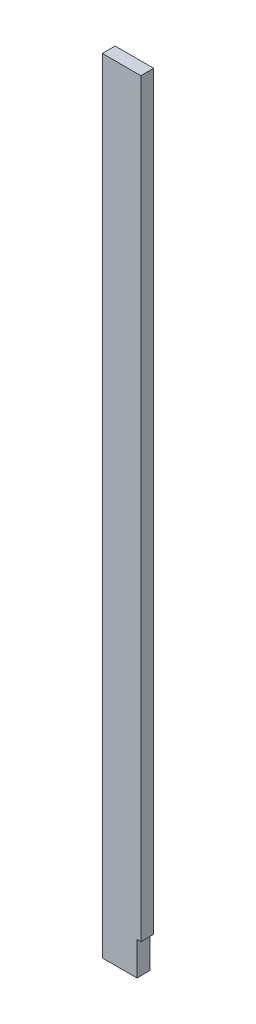
from build123d import *

# Parameters (mm, degrees)
SKETCH1_W           = 30
SKETCH1_H           = 610
BOSS_EXTRUDE1_DEPTH = 10
SKETCH2_W           = 3
SKETCH2_H           = 26
CUT_EXTRUDE1_DEPTH  = 10


with BuildPart() as part:
    # Sketch1 → Boss-Extrude1 (new body)
    with BuildSketch(Plane.XY):
        with Locations((15, -305)):
            Rectangle(SKETCH1_W, SKETCH1_H)
    extrude(amount=BOSS_EXTRUDE1_DEPTH)

    # Sketch2 → Cut-Extrude1 (cut)
    with BuildSketch(Plane.XY.offset(10)):
        with Locations((28.5, -597)):
            Rectangle(SKETCH2_W, SKETCH2_H)
    extrude(amount=-CUT_EXTRUDE1_DEPTH, mode=Mode.SUBTRACT)


solid = part.part
